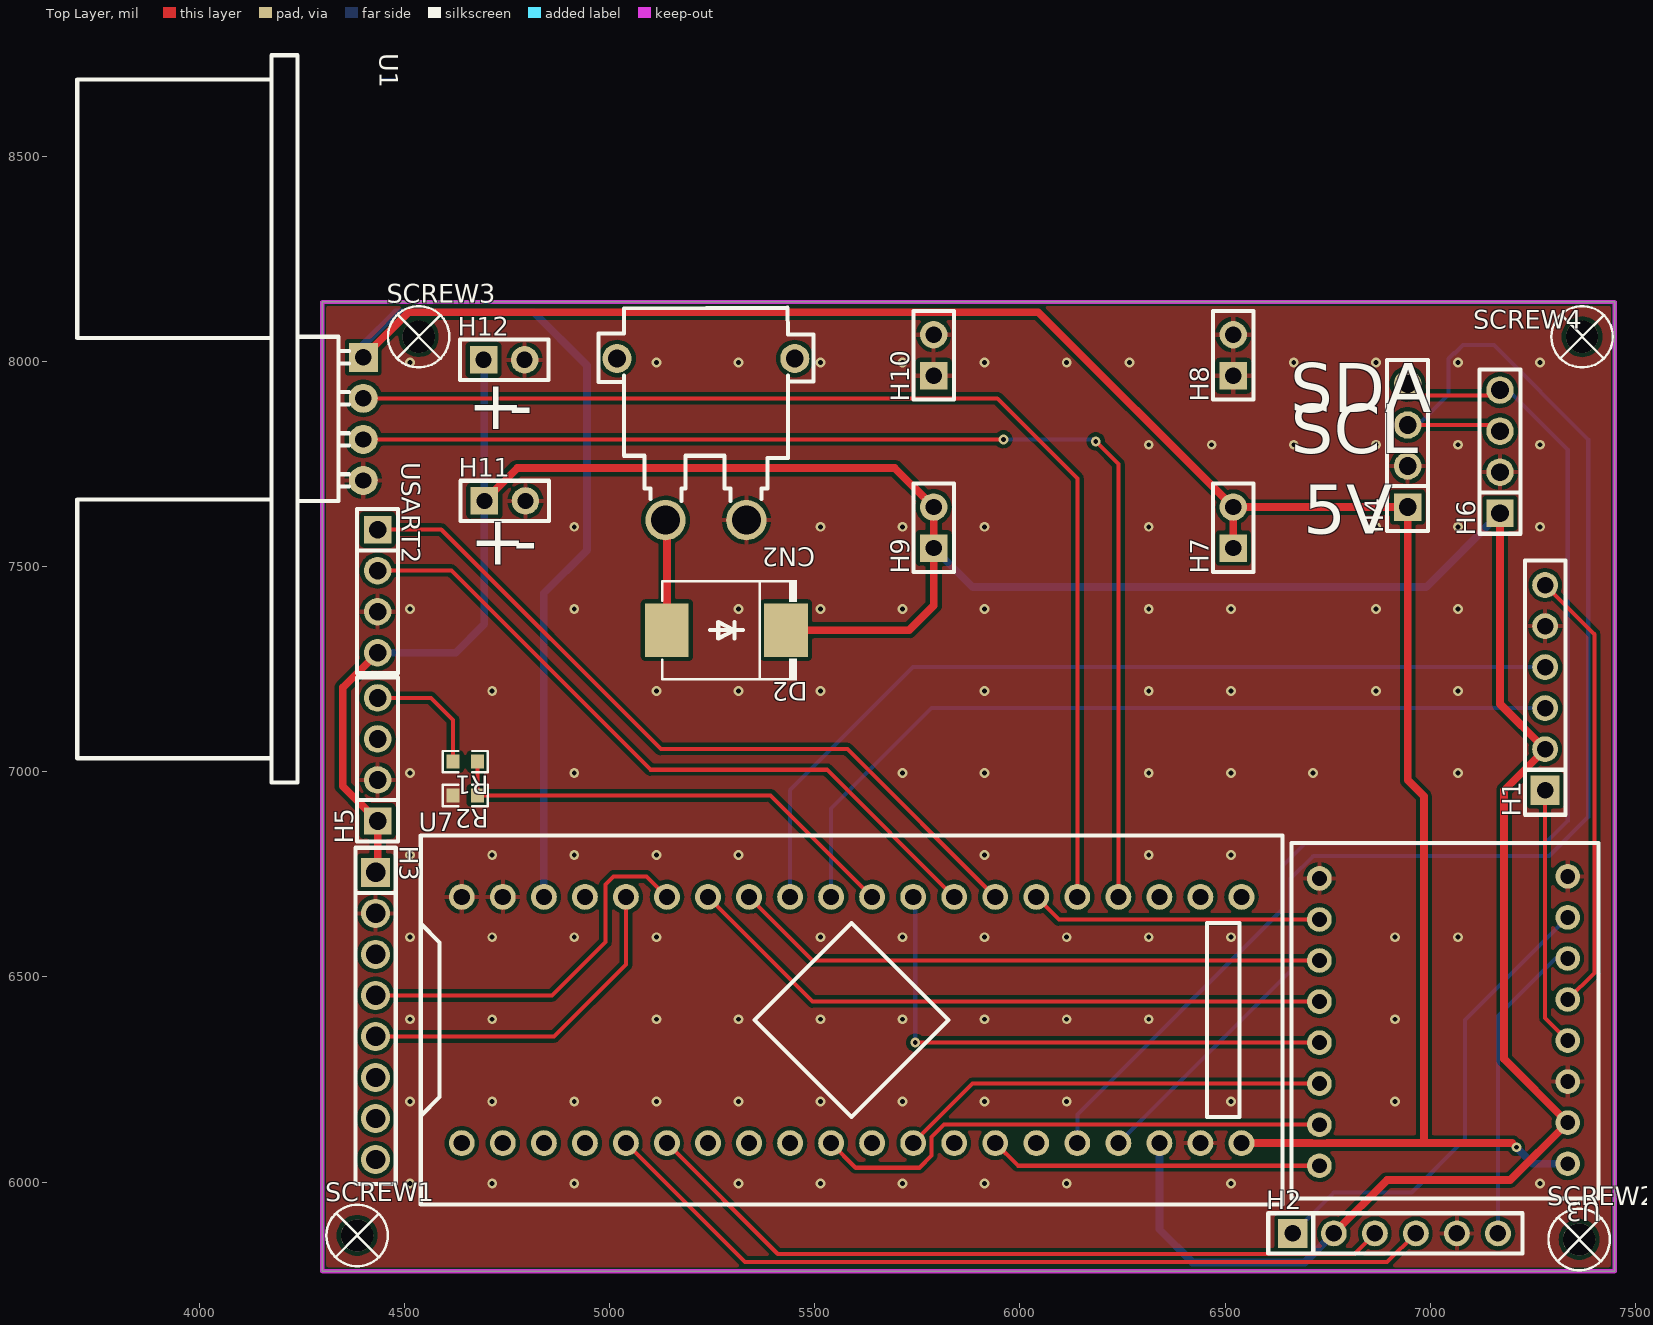
[diagram p0: Top Layer view]
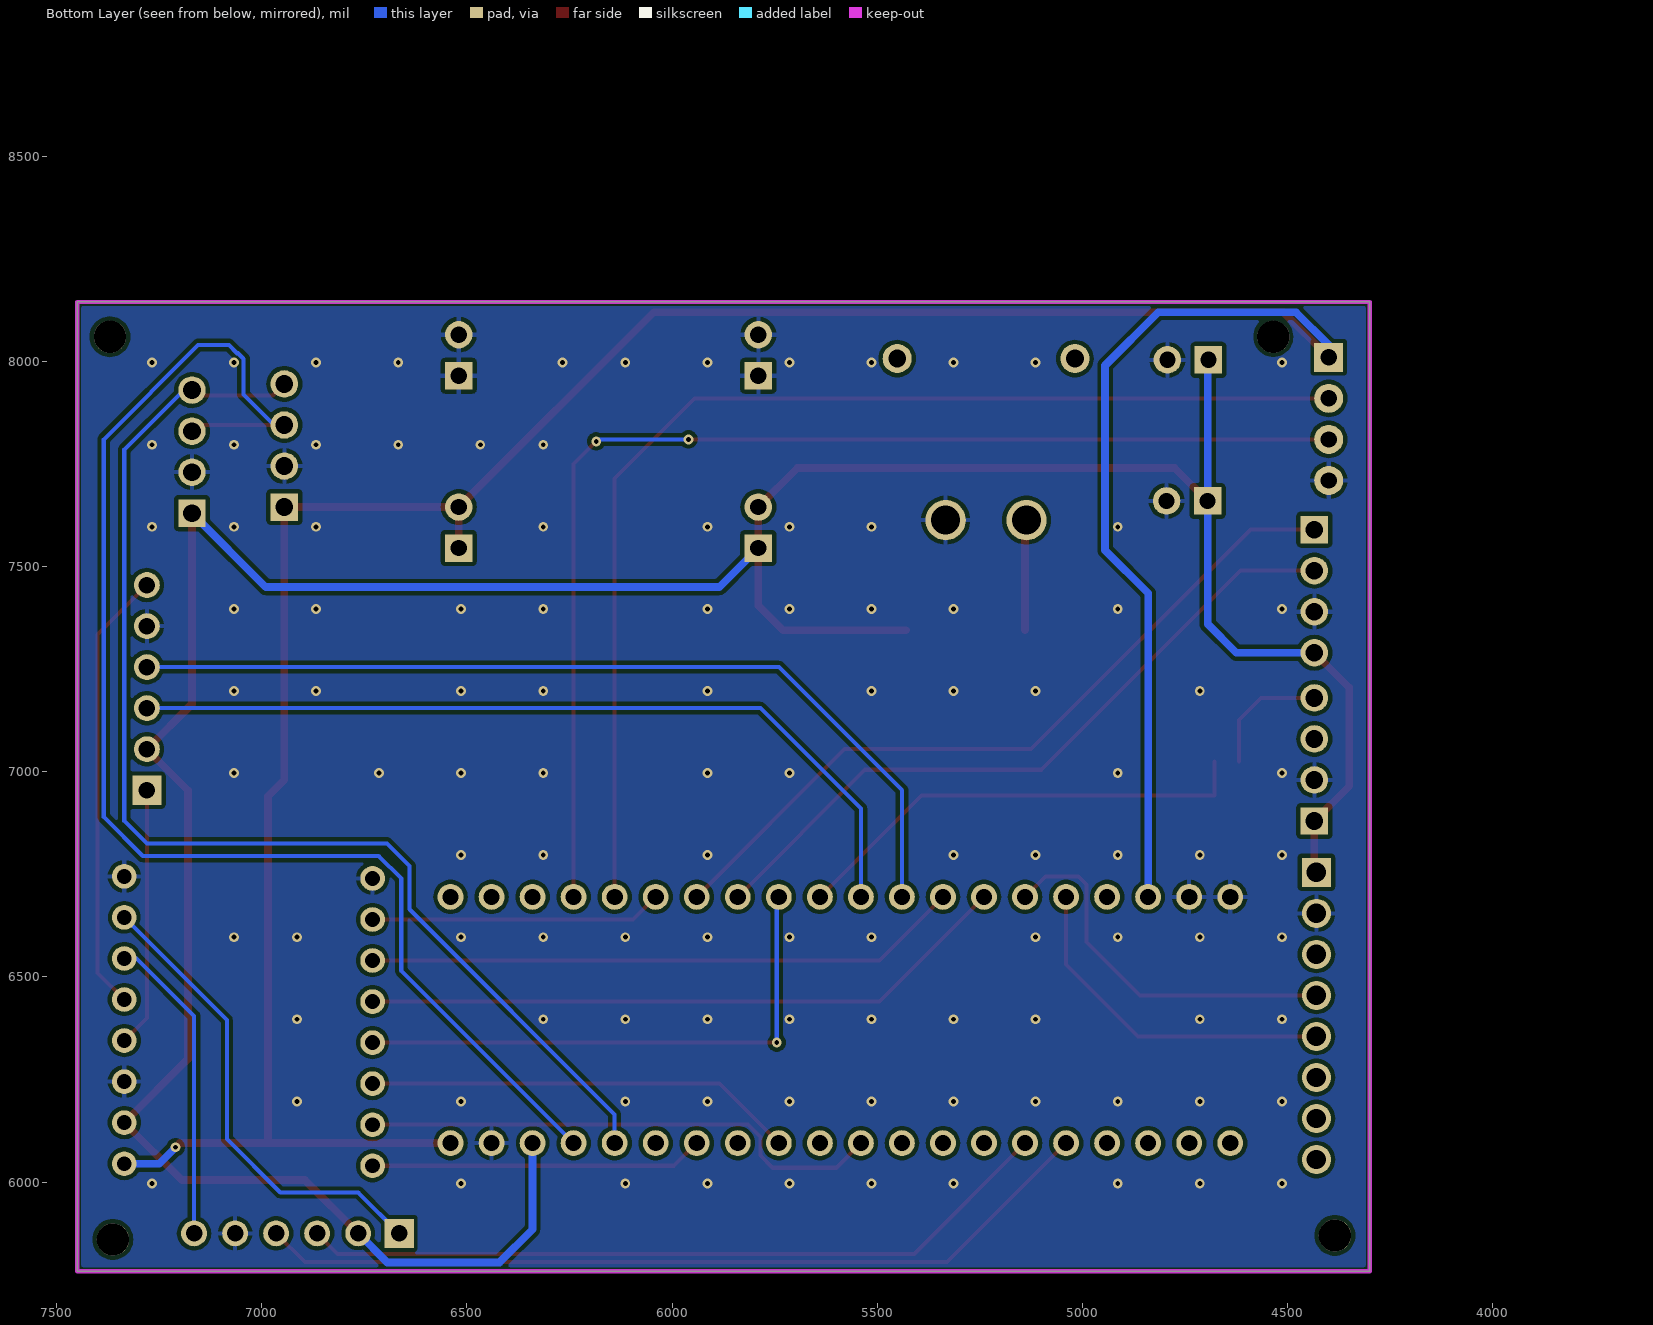
[diagram p1: Bottom Layer view, seen from below]
# Altium PCB MISC52026.pcbdoc
Units mil, origin at the board's own origin, x right, y up, seen from the top; angles counter-clockwise.
Board outline 3149.61 x 2362.2 mil, 2 copper layers (Top Layer, Bottom Layer), stack 62.206 mil thick; 24 components, 29 nets, 122 pads, 108 vias.

## Layer stack, top to bottom
Top Solder Mask Layer: solder mask 0.394, Dk 3.3
Top Layer: signal copper 1.379
Dielectric1: surface 59.449, FR4, Dk 4.5
Bottom Layer: signal copper 1.378
Bottom Solder Mask Layer: solder mask 0.394, Dk 3.3

## Board outline
4300,8145 4300,5782.8 7449.61,5782.8 7449.61,8145

## Design rules (kind name [scope] priority, off if disabled: settings)
BoardOutlineClearance copperThickness2oz_1 [All] p2 off: genericclearance=7.99 ignorepadtopadclearanceinfootprint=FALSE except(0: Arc-SplitContinuation Track-SplitContinuation SMDPad-SplitContinuation THPad-SplitContinuation Via-SplitContinuation Fill-SplitContinuation Region-SplitContinuation Poly-SplitContinuation Text-SplitContinuation Hole-SplitContinuation; 5.98: Arc-CutoutEdge Track-CutoutEdge SMDPad-CutoutEdge THPad-CutoutEdge Via-CutoutEdge Text-CutoutEdge; 6.89: Hole-OutlineEdge Hole-CutoutEdge; 10: Poly-OutlineEdge Poly-CutoutEdge; 11.81: Arc-OutlineEdge Track-OutlineEdge SMDPad-OutlineEdge THPad-OutlineEdge Via-OutlineEdge Fill-OutlineEdge Region-OutlineEdge Text-OutlineEdge Fill-CutoutEdge Region-CutoutEdge)
BoardOutlineClearance Plane_innerPlane_1 [All] p4 off: genericclearance=4.02 ignorepadtopadclearanceinfootprint=FALSE except(0: Arc-SplitContinuation Track-SplitContinuation SMDPad-SplitContinuation THPad-SplitContinuation Via-SplitContinuation Fill-SplitContinuation Region-SplitContinuation Poly-SplitContinuation Text-SplitContinuation Hole-SplitContinuation; 5.98: Arc-CutoutEdge Track-CutoutEdge SMDPad-CutoutEdge THPad-CutoutEdge Via-CutoutEdge Text-CutoutEdge; 6.89: Hole-OutlineEdge Hole-CutoutEdge; 10: Poly-OutlineEdge Poly-CutoutEdge; 11.81: Arc-OutlineEdge Track-OutlineEdge SMDPad-OutlineEdge THPad-OutlineEdge Via-OutlineEdge Fill-OutlineEdge Region-OutlineEdge Text-OutlineEdge Fill-CutoutEdge Region-CutoutEdge)
BoardOutlineClearance Copper_copperRegion_1 [All] p6 off: genericclearance=4.02 ignorepadtopadclearanceinfootprint=FALSE except(0: Arc-SplitContinuation Track-SplitContinuation SMDPad-SplitContinuation THPad-SplitContinuation Via-SplitContinuation Fill-SplitContinuation Region-SplitContinuation Poly-SplitContinuation Text-SplitContinuation Hole-SplitContinuation; 5.98: Arc-CutoutEdge Track-CutoutEdge SMDPad-CutoutEdge THPad-CutoutEdge Via-CutoutEdge Text-CutoutEdge; 6.89: Hole-OutlineEdge Hole-CutoutEdge; 10: Poly-OutlineEdge Poly-CutoutEdge; 11.81: Arc-OutlineEdge Track-OutlineEdge SMDPad-OutlineEdge THPad-OutlineEdge Via-OutlineEdge Fill-OutlineEdge Region-OutlineEdge Text-OutlineEdge Fill-CutoutEdge Region-CutoutEdge)
BoardOutlineClearance copperThickness1oz_1 [All] p8: genericclearance=4.02 ignorepadtopadclearanceinfootprint=FALSE except(0: Arc-SplitContinuation Track-SplitContinuation SMDPad-SplitContinuation THPad-SplitContinuation Via-SplitContinuation Fill-SplitContinuation Region-SplitContinuation Poly-SplitContinuation Text-SplitContinuation Hole-SplitContinuation; 5.98: Arc-CutoutEdge Track-CutoutEdge SMDPad-CutoutEdge THPad-CutoutEdge Via-CutoutEdge Text-CutoutEdge; 6.89: Hole-OutlineEdge Hole-CutoutEdge; 10: Poly-OutlineEdge Poly-CutoutEdge; 11.81: Arc-OutlineEdge Track-OutlineEdge SMDPad-OutlineEdge THPad-OutlineEdge Via-OutlineEdge Fill-OutlineEdge Region-OutlineEdge Text-OutlineEdge Fill-CutoutEdge Region-CutoutEdge)
Clearance copperThickness2oz [All] p1 off: gap=7.99 ignorepadtopadclearanceinfootprint=FALSE except(5.98: SMDPad-Track SMDPad-SMDPad THPad-Track SMDPad-THPad THPad-THPad Track-Via SMDPad-Via THPad-Via Via-Via Fill-SMDPad Region-SMDPad Fill-THPad Region-THPad Fill-Via Region-Via Fill-Fill Fill-Region Region-Region Arc-Track Arc-SMDPad Arc-THPad Arc-Via Fill-Arc Region-Arc Arc-Arc Text-Track SMDPad-Text Text-THPad Text-Via Fill-Text Region-Text Arc-Text Text-Text; 6.89: Hole-Track Hole-SMDPad Hole-THPad Hole-Via Fill-Hole Region-Hole Hole-Arc Hole-Text; 10: Poly-Track Poly-SMDPad Poly-THPad Poly-Via Poly-Fill Poly-Region Poly-Poly Poly-Arc Poly-Text Poly-Hole; 11.81: Fill-Track Region-Track)
Clearance Plane_innerPlane [All] p3 off: gap=4.02 ignorepadtopadclearanceinfootprint=FALSE except(5.98: SMDPad-Track SMDPad-SMDPad THPad-Track SMDPad-THPad THPad-THPad Track-Via SMDPad-Via THPad-Via Via-Via Fill-SMDPad Region-SMDPad Fill-THPad Region-THPad Fill-Via Region-Via Fill-Fill Fill-Region Region-Region Arc-Track Arc-SMDPad Arc-THPad Arc-Via Fill-Arc Region-Arc Arc-Arc Text-Track SMDPad-Text Text-THPad Text-Via Fill-Text Region-Text Arc-Text Text-Text; 6.89: Hole-Track Hole-SMDPad Hole-THPad Hole-Via Fill-Hole Region-Hole Hole-Arc Hole-Text; 10: Poly-Track Poly-SMDPad Poly-THPad Poly-Via Poly-Fill Poly-Region Poly-Poly Poly-Arc Poly-Text Poly-Hole; 11.81: Fill-Track Region-Track)
Clearance Copper_copperRegion [All] p5 off: gap=4.02 ignorepadtopadclearanceinfootprint=FALSE except(5.98: SMDPad-Track SMDPad-SMDPad THPad-Track SMDPad-THPad THPad-THPad Track-Via SMDPad-Via THPad-Via Via-Via Fill-SMDPad Region-SMDPad Fill-THPad Region-THPad Fill-Via Region-Via Fill-Fill Fill-Region Region-Region Arc-Track Arc-SMDPad Arc-THPad Arc-Via Fill-Arc Region-Arc Arc-Arc Text-Track SMDPad-Text Text-THPad Text-Via Fill-Text Region-Text Arc-Text Text-Text; 6.89: Hole-Track Hole-SMDPad Hole-THPad Hole-Via Fill-Hole Region-Hole Hole-Arc Hole-Text; 10: Poly-Track Poly-SMDPad Poly-THPad Poly-Via Poly-Fill Poly-Region Poly-Poly Poly-Arc Poly-Text Poly-Hole; 11.81: Fill-Track Region-Track)
Clearance copperThickness1oz [All] p7: gap=4.02 ignorepadtopadclearanceinfootprint=FALSE except(5.98: SMDPad-Track SMDPad-SMDPad THPad-Track SMDPad-THPad THPad-THPad Track-Via SMDPad-Via THPad-Via Via-Via Fill-SMDPad Region-SMDPad Fill-THPad Region-THPad Fill-Via Region-Via Fill-Fill Fill-Region Region-Region Arc-Track Arc-SMDPad Arc-THPad Arc-Via Fill-Arc Region-Arc Arc-Arc Text-Track SMDPad-Text Text-THPad Text-Via Fill-Text Region-Text Arc-Text Text-Text; 6.89: Hole-Track Hole-SMDPad Hole-THPad Hole-Via Fill-Hole Region-Hole Hole-Arc Hole-Text; 10: Poly-Track Poly-SMDPad Poly-THPad Poly-Via Poly-Fill Poly-Region Poly-Poly Poly-Arc Poly-Text Poly-Hole; 11.81: Fill-Track Region-Track)
DiffPairsRouting differentialPair [All] p1: maxlimit=6 minlimit=6 mostfreqgap=6 toplayer_minwidth=5 toplayer_prefwidth=10 toplayer_maxwidth=100 toplayer_mingap=6 toplayer_prefgap=6 toplayer_maxgap=6 bottomlayer_minwidth=5 bottomlayer_prefwidth=10 bottomlayer_maxwidth=100 bottomlayer_mingap=6 bottomlayer_prefgap=6 bottomlayer_maxgap=6 maxuncoupledlength=10
HoleToHoleClearance otherClearance [All] p1: gap=11.81 allowstackedmicrovias=TRUE
Length netLength [All] p1: minlimit=0 maxlimit=0
PasteMaskExpansion pasteMaskExpansion [All] p1: expansion=0
PlaneConnect innerPlane [All] p1: planeconnectstyle=Relief reliefexpansion=20 reliefentries=4 reliefconductorwidth=10 reliefairgap=10
PolygonConnect copperRegion [All] p1: connectstyle=Relief reliefconductorwidth=10 reliefentries=4 polygonreliefangle="90 Angle" airgapwidth=10 smdpad.connectstyle=Direct via.connectstyle=Relief via.reliefconductorwidth=10 via.reliefentries=4 via.polygonreliefangle="90 Angle" via.airgapwidth=10
RoutingVias viaSize [All] p1: holewidth=12.01 width=24.02 viastyle="Through Hole" minholewidth=11.81 minwidth=19.68 maxholewidth=248.03 maxwidth=393.7
SolderMaskExpansion solderMaskExpansion [IsVia] p1: expansion=-1000 istentingtop=TRUE
SolderMaskExpansion solderMaskExpansion [All] p2: expansion=2.01 istentingtop=FALSE
Width copperThickness2oz_2 [All] p1 off: maxlimit=100 minlimit=8 preferedwidth=10
Width copperThickness1oz_2 [All] p2: maxlimit=100 minlimit=5 preferedwidth=10

## Components (designator, comment, footprint, x,y, rotation, side; value= is the part's Value field where it differs from the comment)
CN2 "XT30PW-M30.G.Y" CONN-TH_XT30PW-M 5235,7810 r180 top
D2 "SS34" SMC_L6.9-W5.9-LS7.9-RD 5285,7345 r180 top
H1 "" HDR-TH_6P-P2.54-V-F 7280,7205 r90 top
H2 "" HDR-TH_6P-P2.54-V-F 6915,5875 r0 top
H3 "" HDR-TH_8P-P2.54-V-F-1 4430,6405 r270 top
H4 "" HDR-TH_4P-P2.54-V-F 6945,7795 r90 top
H5 "" HDR-TH_4P-P2.54-V-M 4435,7030 r90 top
H6 "" HDR-TH_4P-P2.54-V-M 7170,7780 r90 top
H7 "" HDR-TH_2P-P2.54-V-F 6520,7595 r90 top
H8 "" HDR-TH_2P-P2.54-V-F 6520,8015 r90 top
H9 "" HDR-TH_2P-P2.54-V-F 5790,7595 r90 top
H10 "" HDR-TH_2P-P2.54-V-F 5790,8015 r90 top
H11 "" HDR-TH_2P-P2.54-V-F 4745,7660 r0 top
H12 "" HDR-TH_2P-P2.54-V-F 4743.21,8003.84 r0 top
R1 "1K" R0603 4648.38,7024.54 r180 top
R2 "2K" R0603 4648.38,6942.24 r180 top
SCREW1 "" M2螺丝 4385,5870 r0 top
SCREW2 "" M2螺丝 7362.98,5860.25 r0 top
SCREW3 "" M2螺丝 4535,8060 r0 top
SCREW4 "" M2螺丝 7370,8060 r0 top
U1 "HC-SR04" TH_HC-SR04V 4400,7860 r270 top
U3 "" TB6612 6880,8250 r180 top
U7 "LCKFB-DKX-STM32F103C8T6" CONN-TH_L53.3-W22.9_STM32F103C8T6-CARD 5590,6395 r0 top
USART2 "" HDR-TH_4P-P2.54-V-M 4435,7440 r270 top

## Footprints (in the part's own frame and the unit in brackets; to place one, negate y for a bottom-side part, rotate by r counter-clockwise, add the part's x,y. Pads: shape width x height; smd on the part's side, far side on the other; paste and mask are expansions set on the pad)
CONN-TH_L53.3-W22.9_STM32F103C8T6-CARD [mm]
  round 1.6 hole 1: 1(-24.13,-7.62) 2(-21.59,-7.62) 3(-19.05,-7.62) 4(-16.51,-7.62) 5(-13.97,-7.62) 6(-11.43,-7.62) 7(-8.89,-7.62) 8(-6.35,-7.62) 9(-3.81,-7.62) 10(-1.27,-7.62) 11(1.27,-7.62) 12(3.81,-7.62) 13(6.35,-7.62) 14(8.89,-7.62) 15(11.43,-7.62) 16(13.97,-7.62) 17(16.51,-7.62) 18(19.05,-7.62) 19(21.59,-7.62) 20(24.13,-7.62) 21(24.13,7.62) 22(21.59,7.62) 23(19.05,7.62) 24(16.51,7.62) 25(13.97,7.62) 26(11.43,7.62) 27(8.89,7.62) 28(6.35,7.62) 29(3.81,7.62) 30(1.27,7.62) 31(-1.27,7.62) 32(-3.81,7.62) 33(-6.35,7.62) 34(-8.89,7.62) 35(-11.43,7.62) 36(-13.97,7.62) 37(-16.51,7.62) 38(-19.05,7.62) 39(-21.59,7.62) 40(-24.13,7.62)
  silkscreen extent -26.67,-11.43 26.67,11.43
CONN-TH_XT30PW-M [mm]
  round 2.5 hole 1.8: 1(-2.5,5) 2(2.5,5)
  round 1.8 hole 1.1: 3(5.5,-5) 4(-5.5,-5)
  silkscreen extent -6.65,-8.15 6.65,3.81
HDR-TH_2P-P2.54-V-F [mm]
  rect 1.7x1.7 hole 1: 1(-1.27,0)
  round 1.7 hole 1: 2(1.27,0)
  silkscreen extent -2.74,-1.25 2.74,1.25
HDR-TH_4P-P2.54-V-F [mm]
  rect 1.7x1.7 hole 1.1: 1(-3.81,0)
  round 1.7 hole 1.1: 2(-1.27,0) 3(1.27,0) 4(3.81,0)
  silkscreen extent -5.29,-1.27 5.29,1.27
HDR-TH_4P-P2.54-V-M [mm]
  rect 1.7x1.7 hole 1.1: 1(-3.81,0)
  round 1.7 hole 1.1: 2(-1.27,0) 3(1.27,0) 4(3.81,0)
  silkscreen extent -5.08,-1.27 5.08,1.27
HDR-TH_6P-P2.54-V-F [mm]
  rect 1.8x1.8 hole 1.02: 1(-6.35,0)
  round 1.6 hole 1.02: 2(-3.81,0) 3(-1.27,0) 4(1.27,0) 5(3.81,0) 6(6.35,0)
  silkscreen extent -7.87,-1.25 7.87,1.25
HDR-TH_8P-P2.54-V-F-1 [mm]
  rect 1.8x1.8 hole 1.2: 1(-8.89,0)
  round 1.8 hole 1.2: 2(-6.35,0) 3(-3.81,0) 4(-1.27,0) 5(1.27,0) 6(3.81,0) 7(6.35,0) 8(8.89,0)
  silkscreen extent -10.41,-1.25 10.41,1.25
M2螺丝 [mm]
  round 2 hole 2: 1(0,0)
  silkscreen extent -1.9,-1.9 1.9,1.9
R0603 [mil]
  rect 31.75x34.02 smd paste-3937.01 mask+2: 1(-29.66,0) 2(29.66,0)
  silkscreen extent -55,-26 55,26
SMC_L6.9-W5.9-LS7.9-RD [mm]
  rect 2.7x3.3 smd: 1(-3.686,0) 2(3.686,0)
  silkscreen extent -4.36,-3.1 3.98,3.1
TB6612 [mil]
  round 60 hole 36: 1(-455,1505) 2(-455,1605) 3(-455,1705) 4(-455,1805) 5(-455,1905) 6(-455,2005) 7(-455,2105) 8(-455,2205) 9(150,1510) 10(150,1610) 11(150,1710) 12(150,1810) 13(150,1910) 14(150,2010) 15(150,2110) 16(150,2210)
  silkscreen extent -530,1424 218,2290
TH_HC-SR04V [mm]
  rect 1.8x1.8 hole 1.001: 1(-3.81,0)
  round 1.8 hole 1.001: 2(-1.27,0) 3(1.27,0) 4(3.81,0)
  silkscreen extent -22.5,-17.7 22.5,-0.89

## Via types
v1: diameter 24.02, hole 12, Top Layer to Bottom Layer, 108 vias

## Nets (pads, with @x,y where several pads share a name; then routed paths per layer and width w, separated by ;. In a path a pad name is that pad's centre, name@x,y a point inside that pad or via, vN(x,y) a via of type N, cw(c..) or ccw(c..) an arc to the next point about the centre after c; other vN are vias at no path point)
$1N17256: H5.4 R1.2 | length 307.7
  Top Layer w10: H5.4 4565,7180 4618.72,7126.28 R1.2
+5V: D2.1 H1.2 H2.2 H3.1 H5.1 H6.1 H9.1 H9.2 H11.1 H12.1 U3.7 U7.18 USART2.4 | length 7843.1
  Top Layer w19: H3.1 4435,6760 H5.1 4350,6965 4350,7205 USART2.4 ; H11.1 4775,7740 5695,7740 H9.2 H9.1 5790,7405 5730,7345 D2.1 ; H2.2 6895,6005 7195,6005 U3.7 7180,6300 7180,6955 H1.2 7170,7165 H6.1
  Bottom Layer w19: USART2.4 4625,7290 4695,7360 H11.1 4695,8002.05 H12.1 ; H9.1 5885,7450 6990,7450 H6.1 ; U7.18 6340,5885 6420.89,5804.11 6694.11,5804.11 H2.2
+5VT: CN2.2 D2.2 | length 269.5
  Top Layer w19: CN2.2 5139.87,7609.85 D2.2
AN1: U3.14 U7.12 | length 1050.1
  Top Layer w10: U7.12 5885,6240 U3.14
AN2: U3.15 U7.10 | length 1284.7
  Top Layer w10: U7.10 5600,6035 5755,6035 5785,6065 5785,6110 5815,6140 U3.15
BM1A: H1.3 U7.31 | length 2056.5
  Bottom Layer w10: U7.31 5540,6910 5785,7155 H1.3
BM1B: H1.4 U7.32 | length 2224.3
  Bottom Layer w10: U7.32 5440,6955 5740,7255 H1.4
BM2A: H2.3 U7.6 | length 1857.5
  Top Layer w10: U7.6 5410,5825 6815,5825 H2.3
BM2B: H2.4 U7.5 | length 2074.1
  Top Layer w10: U7.5 5330,5805 6895,5805 H2.4
BN1: U3.12 U7.34 | length 1595.6
  Top Layer w10: U7.34 5495,6440 U3.12
BN2: U3.11 U7.33 | length 1454.2
  Top Layer w10: U7.33 5495,6540 U3.11
D1+: H1.6 U3.4 | length 1086.6
  Top Layer w10: H1.6 7400,7335 7400,6510 U3.4
D1-: H1.1 U3.5 | length 632.8
  Top Layer w10: H1.1 7280,6400 U3.5
D2+: H2.6 U3.3 | length 758
  Bottom Layer w10: H2.6 7165,6405 7305,6545 U3.3
D2-: H2.1 U3.2 | length 1158.8
  Bottom Layer w10: H2.1 6765,5975 6955,5975 7085,6105 7085,6395 U3.2
GND: CN2.1 H1.5 H2.5 H3.2 H4.2 H5.2 H6.2 H8.1 H8.2 H10.1 H10.2 H11.2 H12.2 R2.2 U1.4 U3.1 U3.6 U3.9 U7.19 U7.39 U7.40 USART2.3
  other v1: 4514.1,5996.9 4714.1,5996.9 4914.1,5996.9 5314.1,5996.9 5514.1,5996.9 5714.1,5996.9 5914.1,5996.9 6114.1,5996.9 6514.1,5996.9 7267.47,5996.9 4514.1,6196.9 4714.1,6196.9 4914.1,6196.9 5114.1,6196.9 5314.1,6196.9 5514.1,6196.9 5714.1,6196.9 5914.1,6196.9 6114.1,6196.9 6514.1,6196.9 6914.1,6196.9 4514.1,6396.9 4714.1,6396.9 5114.1,6396.9 5314.1,6396.9 5514.1,6396.9 5714.1,6396.9 5914.1,6396.9 6114.1,6396.9 6314.1,6396.9 6914.1,6396.9 4514.1,6596.9 4714.1,6596.9 4914.1,6596.9 5114.1,6596.9 5514.1,6596.9 5714.1,6596.9 5914.1,6596.9 6114.1,6596.9 6314.1,6596.9 6514.1,6596.9 6914.1,6596.9 7067.47,6596.9 4514.1,6796.9 4714.1,6796.9 4914.1,6796.9 5114.1,6796.9 5314.1,6796.9 5914.1,6796.9 6314.1,6796.9 6514.1,6796.9 4514.1,6996.9 4914.1,6996.9 5714.1,6996.9 5914.1,6996.9 6314.1,6996.9 6514.1,6996.9 6714.1,6996.9 7067.47,6996.9 4714.1,7196.9 5114.1,7196.9 5314.1,7196.9 5514.1,7196.9 5914.1,7196.9 6314.1,7196.9 6514.1,7196.9 6867.47,7196.9 7067.47,7196.9 4514.1,7396.9 4914.1,7396.9 5314.1,7396.9 5514.1,7396.9 5714.1,7396.9 5914.1,7396.9 6314.1,7396.9 6514.1,7396.9 6867.47,7396.9 7067.47,7396.9 4914.1,7596.9 5514.1,7596.9 5714.1,7596.9 5914.1,7596.9 6314.1,7596.9 6867.47,7596.9 7067.47,7596.9 7267.47,7596.9 6314.1,7796.9 6467.47,7796.9 6667.47,7796.9 6867.47,7796.9 7067.47,7796.9 7267.47,7796.9 4514.1,7996.9 5114.1,7996.9 5314.1,7996.9 5514.1,7996.9 5714.1,7996.9 5914.1,7996.9 6114.1,7996.9 6267.47,7996.9 6667.47,7996.9 6867.47,7996.9 7067.47,7996.9 7267.47,7996.9
PA0: U1.2 U7.25 | length 2840.8
  Top Layer w10: U1.2 5945,7910 6140,7715 U7.25
PA5: R1.1 R2.1 U7.30 | length 1146.7
  Top Layer w10: R1.1 R2.1 5392.77,6942.24 U7.30
PB10: H3.4 U7.35 | length 932.8
  Top Layer w10: H3.4 4860,6455 4990,6585 4990,6725 5010,6745 5090,6745 U7.35
PB11: H3.5 U7.36 | length 847.5
  Top Layer w10: H3.5 4865,6355 5040,6530 U7.36
PC15: U1.3 U7.24 | length 2919.9
  Top Layer w10: U1.3 v1(5960,7810) ; v1(6185,7805) 6240,7750 U7.24
  Bottom Layer w10: v1(5960,7810) 6180,7810 v1(6185,7805)
PWMA: U3.16 U7.14 | length 812.8
  Top Layer w10: U7.14 5995,6040 U3.16
PWMB: U3.10 U7.26 | length 712.8
  Top Layer w10: U7.26 6095,6640 U3.10
RX: U7.28 USART2.2 | length 1734.3
  Top Layer w10: USART2.2 4615,7490 5100,7005 5530,7005 U7.28
SCL: H4.4 H6.4 U7.16 | length 2994.9
  Top Layer w10: H4.4 6973.22,7916.78 7156.78,7916.78 H6.4
  Bottom Layer w10: U7.16 6140,6165 6640,6665 6640,6770 6695,6825 7280,6825 7335,6880 7335,7785 7190,7930 H6.4
SDA: H4.3 H6.3 U7.17 | length 3424.3
  Top Layer w10: H4.3 7155,7845 H6.3
  Bottom Layer w10: U7.17 6660,6515 6660,6740 6715,6795 7290,6795 7385,6890 7385,7810 7155,8040 7080,8040 7059.89,8019.89 7057.95,8019.89 7044.48,8006.42 7044.48,7919.48 6970,7845 H4.3
ST: U3.13 U7.29 | length 1342.1
  Top Layer w10: v1(5745,6340) U3.13
  Bottom Layer w10: U7.29 5745,6690 v1(5745,6340)
TX: U7.27 USART2.1 | length 1875.7
  Top Layer w10: USART2.1 4590,7590 5125,7055 5580,7055 U7.27
VCC: H4.1 H7.1 H7.2 U1.1 U3.8 U7.20 U7.38 | length 7270.4
  Top Layer w19: U1.1 4510,8120 6045,8120 H7.2 ; H7.1 H7.2 ; U7.20 6710.67,6095 6711.16,6094.52 6748.84,6094.52 6749.33,6095 6984.72,6095 ; v1(7210,6085) 7200,6095 6984.72,6095 ; H7.2 H4.1 6945,6980 6984.72,6940.28 6984.72,6095
  Bottom Layer w19: U1.1 4400,8040 4480,8120 4815,8120 4945,7990 4945,7540 4840,7435 U7.38 ; v1(7210,6085) 7250,6045 U3.8
pads on no net: CN2.3 CN2.4 H3.3 H3.6 H3.7 H3.8 H5.3 SCREW1.1 SCREW2.1 SCREW3.1 SCREW4.1 U7.1 U7.2 U7.3 U7.4 U7.7 U7.8 U7.9 U7.11 U7.13 U7.15 U7.21 U7.22 U7.23 U7.37

## Polygon pours and split planes (outlines as drawn)
GND on Top Layer (solid, remove dead copper, pour order 0): 3000,8835 3000,3000 9330,3000 9330,8835
GND on Bottom Layer (solid, remove dead copper, pour order 2): 3625,8800 3625,3490 8730,3490 8730,8800

## Keep-outs
Board Outline Layer:
  the board outline again, w10

## Silkscreen, mask and mechanical layers (free items; w line width, h text height)
Top Silkscreen Layer:
  text "SDA" at 6659.2,7875.8 h120
  text "+" at 4655,7835 h120
  text "-" at 4755,7835 h120
  text "SCL" at 6659.7,7775.8 h120
  text "5V" at 6690,7580 h120
  text "+" at 4660,7505 h120
  text "-" at 4765,7505 h120